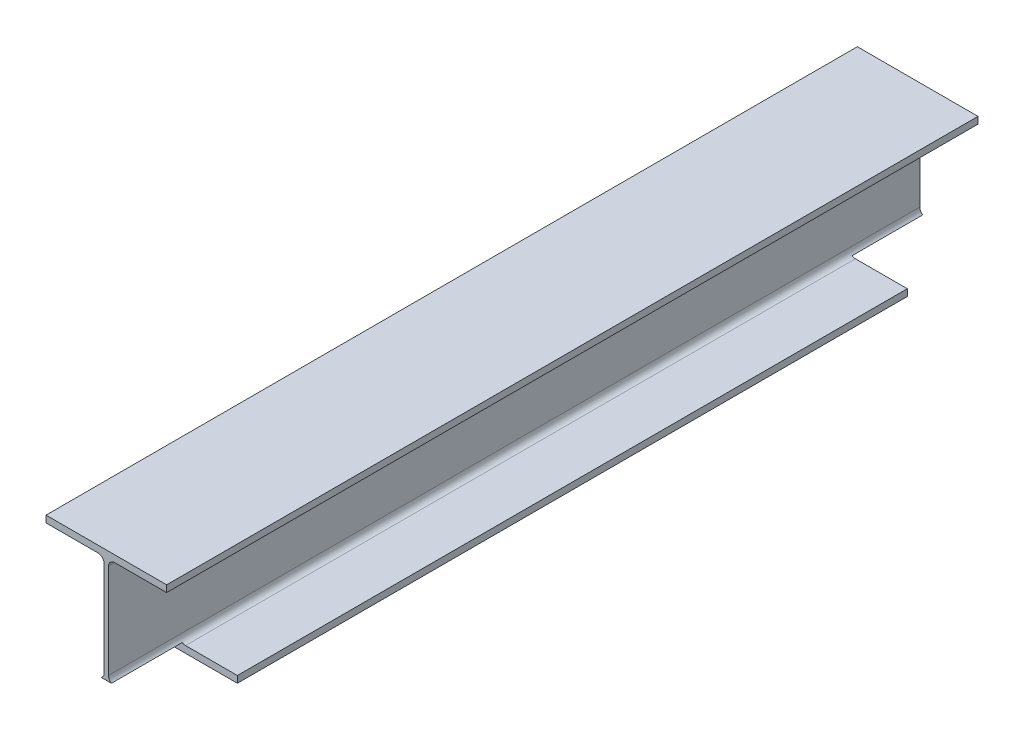
SolidWorks part; units mm, degrees
material "Q235"
ref_plane "Front Plane" through (0, 0, 0) normal (0, 0, 1) x (1, 0, 0)
ref_plane "Top Plane" through (0, 0, 0) normal (0, 1, 0) x (1, 0, 0)
ref_plane "Right Plane" through (0, 0, 0) normal (1, 0, 0) x (0, 0, -1)
sketch "Sketch1" plane through (0, 0, 0) normal (0, 0, 1) x (1, 0, 0)
  line L0 (0, 0) -> (250, 0)
  line L1 (250, 0) -> (250, 14)
  line L2 (250, 14) -> (142.5, 14)
  line L3 (129.5, 27) -> (129.5, 223)
  line L4 (142.5, 236) -> (250, 236)
  line L5 (250, 236) -> (250, 250)
  line L6 (250, 250) -> (0, 250)
  line L7 (0, 250) -> (0, 236)
  line L8 (0, 236) -> (107.5, 236)
  line L9 (120.5, 223) -> (120.5, 27)
  line L10 (107.5, 14) -> (0, 14)
  line L11 (0, 14) -> (0, 0)
  line L12 (125, 250) -> (125, 0) construction
  arc A0 (142.5, 14) -> (129.5, 27) centre (142.5, 27) cw
  arc A1 (120.5, 27) -> (107.5, 14) centre (107.5, 27) cw
  arc A2 (129.5, 223) -> (142.5, 236) centre (142.5, 223) cw
  arc A3 (107.5, 236) -> (120.5, 223) centre (107.5, 223) cw
  point P21 (129.5, 236)
  dimension "D7" = 13
  dimension "D1" = 250
  dimension "D2" = 250
  dimension "D3" = 9
  dimension "D4" = 4.5
  dimension "D5" = 14
  dimension "D6" = 14
extrude "Boss-Extrude1" add sketch "Sketch1" along normal blind 1681
sketch "Sketch2" plane through (0, 250, 0) normal (0, 1, 0) x (1, 0, 0)
  line L0 (125, -1681) -> (125, 0) construction
  line L1 (250, -1681) -> (0, -1681) construction
  line L2 (250, 0) -> (0, 0) construction
sketch "Sketch3" plane through (0, 0, 0) normal (0, -1, 0) x (-1, 0, 0)
  line L0 (0, -1681) -> (0, 0) construction
  line L1 (-250, 0) -> (0, 0)
  line L2 (-250, 0) -> (-250, -146.5)
  line L3 (-250, -146.5) -> (0, -146.5)
  line L4 (0, 0) -> (0, -146.5)
  line L6 (-250, -1681) -> (0, -1681)
  line L7 (-250, -1681) -> (-250, -1534.5)
  line L8 (-250, -1534.5) -> (0, -1534.5)
  line L9 (0, -1681) -> (0, -1534.5)
  dimension "D1" = 146.5
  dimension "D2" = 146.5
extrude "Cut-Extrude1" cut sketch "Sketch3" against normal blind 16
